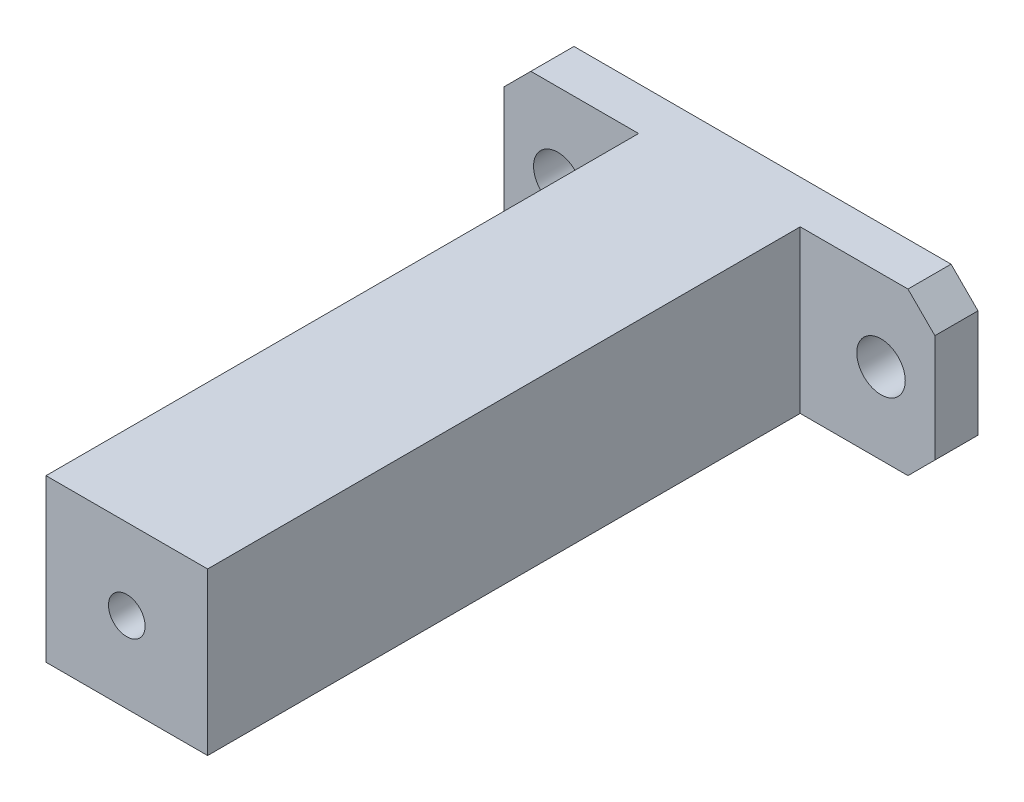
SolidWorks part; units mm, degrees
ref_plane "Front Plane" through (0, 0, 0) normal (0, 0, 1) x (1, 0, 0)
ref_plane "Top Plane" through (0, 0, 0) normal (0, 1, 0) x (1, 0, 0)
ref_plane "Right Plane" through (0, 0, 0) normal (1, 0, 0) x (0, 0, -1)
sketch "Sketch1" plane through (0, 0, 0) normal (0, 0, 1) x (1, 0, 0)
  line L0 (-40, 10) -> (-35, 15)
  line L1 (35, -15) -> (-35, -15)
  line L2 (40, -10) -> (40, 10)
  line L3 (35, 15) -> (-35, 15)
  line L4 (-40, -10) -> (-40, 10)
  line L5 (40, -15) -> (-40, 15) construction
  line L6 (40, 15) -> (-40, -15) construction
  line L7 (40, 10) -> (35, 15)
  line L8 (35, -15) -> (40, -10)
  line L9 (-35, -15) -> (-40, -10)
  line L10 (-40, 0) -> (40, 0) construction
  line L11 (0, 15) -> (0, -41.8993) construction
  circle A0 centre (-30, 0) radius 4.5
  circle A1 centre (30, 0) radius 4.5
  point P0 (0, 0)
  dimension "D3" = 9
  dimension "D4" = 10
  dimension "D5" = 10
  dimension "D1" = 30
  dimension "D2" = 80
extrude "Boss-Extrude1" add sketch "Sketch1" along normal blind 8
sketch "Sketch2" plane through (0, 0, 8) normal (0, 0, 1) x (1, 0, 0)
  line L0 (35, 15) -> (-35, 15) construction
  line L1 (15, -15) -> (-15, -15)
  line L2 (15, -15) -> (15, 15)
  line L3 (15, 15) -> (-15, 15)
  line L4 (-15, -15) -> (-15, 15)
  line L5 (15, -15) -> (-15, 15) construction
  line L6 (15, 15) -> (-15, -15) construction
  point P0 (0, 0)
  dimension "D1" = 30
extrude "Boss-Extrude2" add sketch "Sketch2" along normal blind 110
sketch "Sketch3" plane through (0, 0, 118) normal (0, 0, 1) x (1, 0, 0)
  circle A0 centre (0, 0) radius 1.5
  dimension "D1" = 3
extrude "Cut-Extrude1" cut sketch "Sketch3" against normal blind 10
hole_wizard "M8 Tapped Hole1" positions "3DSketch1" profile "Sketch4" tap size "M8" standard "GB"
sketch3d "3DSketch1"
  line L0 (0, 0, 108) -> (0, 0, 118) construction
  point P0 (0, 0, 118)
sketch "Sketch4" plane through (0, 0, 118) normal (1, 0, 0) x (0, -1, 0)
  line L0 (0, 0) -> (0, 27.0429)
  line L1 (0, 27.0429) -> (3.4, 25)
  line L2 (3.4, 25) -> (3.4, 0)
  line L5 (3.4, 0) -> (0, 0)
  line L10 (0, 27.0429) -> (-3.4, 25) construction
  line L11 (0, -6.35) -> (0, 107.95) construction
  dimension "螺纹孔钻头直径" = 6.8
  dimension "螺纹孔钻头深度" = 25
  dimension "导头角度" = 118
cosmetic thread "Hole thread1" parameters "D1"=16, "D2"=8
